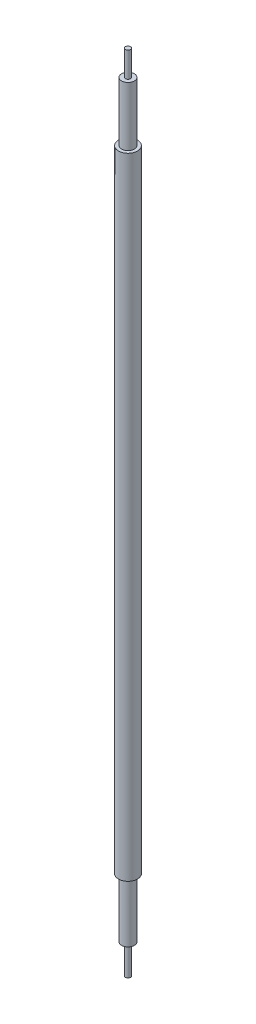
SolidWorks part; units mm, degrees
material "铜"
ref_plane "Front Plane" through (0, 0, 0) normal (0, 0, 1) x (1, 0, 0)
ref_plane "Top Plane" through (0, 0, 0) normal (0, 1, 0) x (1, 0, 0)
ref_plane "Right Plane" through (0, 0, 0) normal (1, 0, 0) x (0, 0, -1)
sketch "Sketch1" plane through (0, 0, 0) normal (0, 1, 0) x (1, 0, 0)
  circle A0 centre (0, 0) radius 1.125
extrude "Boss-Extrude1" add sketch "Sketch1" along normal blind 74.7
sketch "Sketch2" plane through (0, 0, 0) normal (0, -1, 0) x (1, 0, 0)
  circle A0 centre (0, 0) radius 0.75
  dimension "D1" = 1.5
extrude "Boss-Extrude2" add sketch "Sketch2" along normal blind 7
sketch "Sketch3" plane through (0, -7, 0) normal (0, -1, 0) x (1, 0, 0)
  circle A0 centre (0, 0) radius 0.3
  dimension "D1" = 0.6
extrude "Boss-Extrude3" add sketch "Sketch3" along normal blind 3.5
sketch "Sketch4" plane through (0, 74.7, 0) normal (0, 1, 0) x (1, 0, 0)
  circle A0 centre (0, 0) radius 0.75
  circle A4 centre (0, 0) radius 0.75 construction
extrude "Boss-Extrude4" add sketch "Sketch4" along normal blind 7
sketch "Sketch5" plane through (0, 81.7, 0) normal (0, 1, 0) x (1, 0, 0)
  circle A0 centre (0, 0) radius 0.2999
extrude "Boss-Extrude5" add sketch "Sketch5" along normal blind 3
